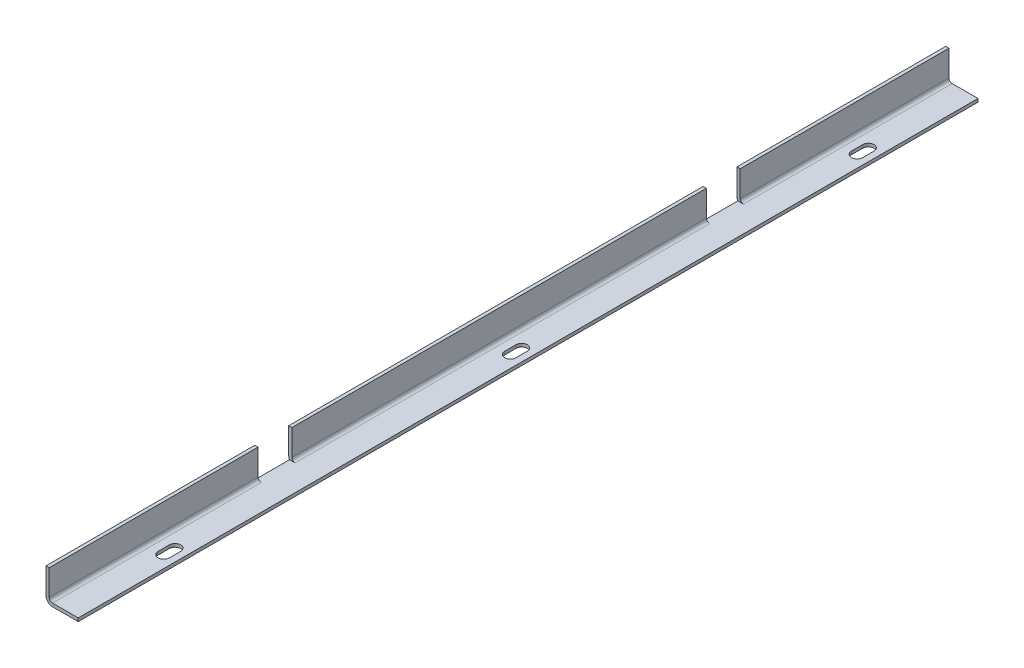
from build123d import *

# Parameters (mm, degrees)
EXTRUDE_THIN1_DEPTH = 1116
SKETCH2_W           = 42
SKETCH2_H           = 50
CUT_EXTRUDE1_DEPTH  = 1118.432772027
CUT_EXTRUDE2_DEPTH  = 10
LPATTERN1_COUNT     = 2
LPATTERN1_PITCH     = 430
LPATTERN2_COUNT     = 2
LPATTERN2_PITCH     = 430


with BuildPart() as part:
    # Sketch1 → Extrude-Thin1 (new body)
    with BuildSketch(Plane.XY):
        with BuildLine():
            Line((40, 0), (8, 0))
            ThreePointArc((8, 0), (2.343145751, 2.343145751), (0, 8))
            Line((0, 8), (0, 40))
            Line((0, 40), (4, 40))
            Line((4, 40), (4, 8))
            ThreePointArc((4, 8), (5.171572875, 5.171572875), (8, 4))
            Line((8, 4), (40, 4))
            Line((40, 4), (40, 0))
        make_face()
    extrude(amount=EXTRUDE_THIN1_DEPTH)

    # Sketch2 → Cut-Extrude1 (cut, through all)
    with BuildSketch(Plane(origin=(40, 0, 0), x_dir=(0, 0, -1), z_dir=(1, 0, 0))):
        with Locations((-280, 29)):
            Rectangle(SKETCH2_W, SKETCH2_H)
        with Locations((-836, 29)):
            Rectangle(SKETCH2_W, SKETCH2_H)
    extrude(amount=-CUT_EXTRUDE1_DEPTH, mode=Mode.SUBTRACT)

    # Sketch3 → Cut-Extrude2 (cut)
    with BuildSketch(Plane(origin=(0, 4, 0), x_dir=(1, 0, 0), z_dir=(0, 1, 0))):
        with BuildLine():
            Line((32, -551), (32, -565))
            ThreePointArc((32, -565), (25, -572), (18, -565))
            Line((18, -565), (18, -551))
            ThreePointArc((18, -551), (25, -544), (32, -551))
        make_face()
    cut_extrude2 = extrude(amount=-CUT_EXTRUDE2_DEPTH, mode=Mode.SUBTRACT)

    # LPattern1: Cut-Extrude2 ×2
    with Locations(*[(0, 0, -i * LPATTERN1_PITCH) for i in range(1, LPATTERN1_COUNT)]):
        add(cut_extrude2, mode=Mode.SUBTRACT)

    # LPattern2: Cut-Extrude2 ×2
    with Locations(*[(0, 0, i * LPATTERN2_PITCH) for i in range(1, LPATTERN2_COUNT)]):
        add(cut_extrude2, mode=Mode.SUBTRACT)


solid = part.part
